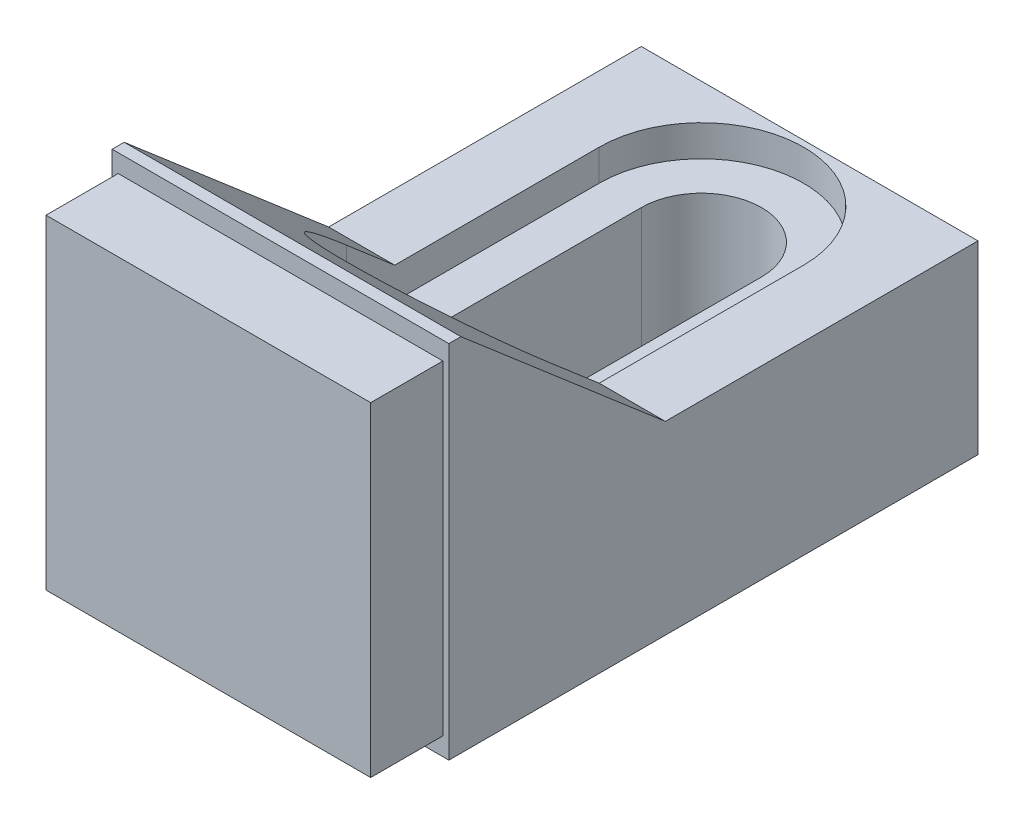
SolidWorks part; units mm, degrees
ref_plane "Front Plane" through (0, 0, 0) normal (0, 0, 1) x (1, 0, 0)
ref_plane "Top Plane" through (0, 0, 0) normal (0, 1, 0) x (1, 0, 0)
ref_plane "Right Plane" through (0, 0, 0) normal (1, 0, 0) x (0, 0, -1)
sketch "Sketch1" plane through (0, 0, 0) normal (0, 0, 1) x (1, 0, 0)
  line L1 (-6.75, 6.75) -> (6.75, 6.75)
  line L2 (-6.75, 6.75) -> (-6.75, -6.75)
  line L3 (-6.75, -6.75) -> (6.75, -6.75)
  line L4 (6.75, 6.75) -> (6.75, -6.75)
  line L5 (0, -6.75) -> (0, 6.75) construction
  line L6 (-6.75, 0) -> (6.75, 0) construction
  point P0 (0, 0)
  dimension "D1" = 13.5
  dimension "D2" = 13.5
extrude "Boss-Extrude1" add sketch "Sketch1" along normal mid plane 3
sketch "Sketch2" plane through (0, 0, -1.5) normal (0, 0, -1) x (-1, 0, 0)
  line L1 (-7, 7.5) -> (7, 7.5)
  line L2 (-7, 7.5) -> (-7, -7.5)
  line L3 (-7, -7.5) -> (7, -7.5)
  line L4 (7, 7.5) -> (7, -7.5)
  line L5 (0, -7.5) -> (0, 7.5) construction
  line L6 (-7, 0) -> (7, 0) construction
  point P0 (0, 0)
  dimension "D1" = 14
  dimension "D2" = 15
extrude "Boss-Extrude2" add sketch "Sketch2" along normal blind 22
sketch "Sketch3" plane through (7, 0, 0) normal (1, 0, 0) x (0, 0, -1)
  line L0 (23.5, -7.5) -> (23.5, 0.2) construction
  line L1 (23.5, 7.5) -> (23.5, -7.5) construction
  line L2 (23.5, 0.2) -> (10.5, 0.2)
  line L3 (10.5, 0.2) -> (2, 7.5)
  line L4 (23.5, 7.5) -> (1.5, 7.5) construction
  dimension "D1" = 7.7
  dimension "D2" = 13
  dimension "D3" = 0.5
extrude "Cut-Extrude2" cut sketch "Sketch3" against normal through all and the other way through all flip side to cut
sketch "Sketch4" plane through (0, 0.2, 0) normal (0, 1, 0) x (1, 0, 0)
  line L0 (0, 23.5) -> (0, 1.5) construction
  line L1 (7, 23.5) -> (-7, 23.5) construction
  line L2 (6.75, 1.5) -> (-6.75, 1.5) construction
  line L3 (0, 19) -> (0, 8.5) construction
  line L4 (4.25, 19) -> (4.25, 8.5)
  line L5 (-4.25, 19) -> (-4.25, 8.5)
  line L6 (0, 19) -> (0, 8.5) construction
  line L7 (2.5, 19) -> (2.5, 8.5)
  line L8 (-2.5, 19) -> (-2.5, 8.5)
  arc A0 (4.25, 19) -> (-4.25, 19) centre (0, 19) ccw
  arc A1 (-4.25, 8.5) -> (4.25, 8.5) centre (0, 8.5) ccw
  arc A2 (2.5, 19) -> (-2.5, 19) centre (0, 19) ccw
  arc A3 (-2.5, 8.5) -> (2.5, 8.5) centre (0, 8.5) ccw
  point P8 (0, 13.75)
  point P15 (0, 13.75)
  dimension "D1" = 4.25
  dimension "D4" = 2.5
  dimension "D2" = 15
  dimension "D3" = 4.5
sketch "Sketch5" plane through (0, 7.5, 0) normal (0, 1, 0) x (1, 0, 0)
  line L0 (-4.25, 19) -> (-4.25, 8.5) construction
  line L1 (-4.25, 19) -> (-4.25, 8.5)
  line L2 (4.25, 19) -> (4.25, 8.5) construction
  line L3 (4.25, 19) -> (4.25, 8.5)
  line L4 (-2.5, 19) -> (-2.5, 8.5) construction
  line L5 (-2.5, 19) -> (-2.5, 8.5)
  line L6 (2.5, 19) -> (2.5, 8.5) construction
  line L7 (2.5, 19) -> (2.5, 8.5)
  arc A0 (-2.5, 8.5) -> (2.5, 8.5) centre (0, 8.5) ccw construction
  arc A1 (-4.25, 8.5) -> (4.25, 8.5) centre (0, 8.5) ccw construction
  arc A2 (-2.5, 8.5) -> (2.5, 8.5) centre (0, 8.5) ccw
  arc A3 (-4.25, 8.5) -> (4.25, 8.5) centre (0, 8.5) ccw
  arc A4 (4.25, 19) -> (-4.25, 19) centre (0, 19) ccw construction
  arc A5 (4.25, 19) -> (-4.25, 19) centre (0, 19) ccw
  arc A6 (2.5, 19) -> (-2.5, 19) centre (0, 19) ccw construction
  arc A7 (2.5, 19) -> (-2.5, 19) centre (0, 19) ccw
extrude "Cut-Extrude3" cut sketch "Sketch5" against normal offset from surface (8.6 mm away) 1.3 contours L1 A3 L3 A5 up to face at (0, 0.2, -17) offset beyond the face yes
extrude "Cut-Extrude4" cut sketch "Sketch4" against normal blind 11.3 contours A3 L7 A2 L8
